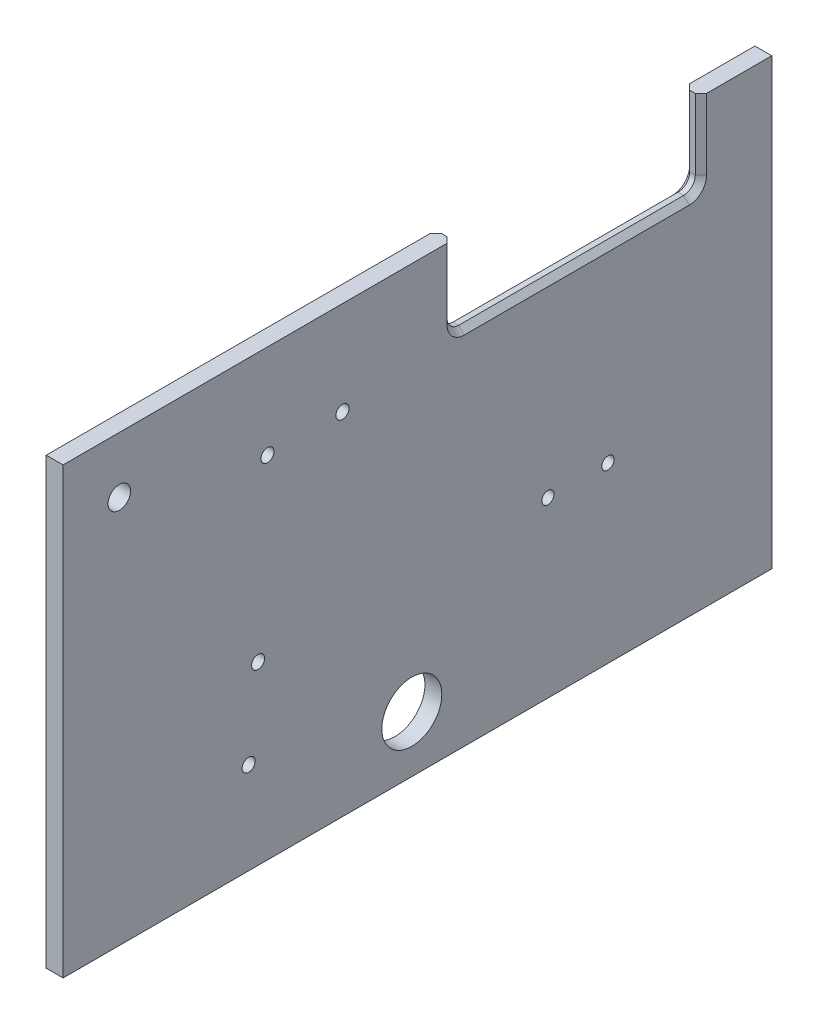
SolidWorks part; units mm, degrees
material "Q235-A"
ref_plane "Front Plane" through (0, 0, 0) normal (0, 0, 1) x (1, 0, 0)
ref_plane "Top Plane" through (0, 0, 0) normal (0, 1, 0) x (1, 0, 0)
ref_plane "Right Plane" through (0, 0, 0) normal (1, 0, 0) x (0, 0, -1)
sketch "Sketch1" plane through (0, 0, 0) normal (1, 0, 0) x (0, 0, -1)
  line L0 (0, -592.4523) -> (0, 592.4523) construction
  line L1 (0, 0) -> (520, 0)
  line L2 (520, 0) -> (520, 1185)
  line L3 (520, 1185) -> (331, 1185)
  line L4 (331, 1185) -> (331, 965)
  line L5 (331, 965) -> (-331, 965)
  line L6 (-331, 965) -> (-331, 1185)
  line L7 (-331, 1185) -> (-1370, 1185)
  line L8 (-1370, 1185) -> (-1370, 0)
  line L9 (-1370, 0) -> (0, 0)
  point P3 (0, 0)
  dimension "D1" = 1185
  dimension "D2" = 1890
  dimension "D3" = 520
  dimension "D4" = 662
  dimension "D5" = 220
extrude "Boss-Extrude1" add sketch "Sketch1" along normal mid plane 45
sketch "Sketch2" plane through (22.5, 0, 0) normal (1, 0, 0) x (0, 0, -1)
  line L0 (-331, 1185) -> (-1370, 1185) construction
  line L1 (-1370, 1185) -> (-1370, 0) construction
  line L2 (0, 0) -> (0, 260.9567) construction
  line L3 (-1370, 0) -> (520, 0) construction
  circle A0 centre (-1220, 1035) radius 30
  circle A1 centre (-825, 935) radius 17.5
  circle A2 centre (-625, 935) radius 17.5
  circle A3 centre (-850, 470) radius 17.5
  circle A4 centre (-875, 245) radius 17.5
  circle A5 centre (-440, 150) radius 80
  dimension "D1" = 150
  dimension "D2" = 150
  dimension "D3" = 60
  dimension "D4" = 495
  dimension "D5" = 25
  dimension "D6" = 25
  dimension "D7" = 200
  dimension "D8" = 35
  dimension "D9" = 250
  dimension "D10" = 465
  dimension "D11" = 225
  dimension "D12" = 440
  dimension "D13" = 150
  dimension "D14" = 160
extrude "Cut-Extrude1" cut sketch "Sketch2" against normal through all
fillet "Fillet1" radius 31 2 edges at (0, 965, -331) (0, 965, 331)
chamfer "Chamfer1" distance 15 angle 45 10 edges at (-22.5, 1090.5, 331) (-22.5, 974.0797, 321.9203) (-22.5, 965, 0) (-22.5, 974.0797, -321.9203) (-22.5, 1090.5, -331) (22.5, 1090.5, -331) (22.5, 974.0797, -321.9203) (22.5, 965, 0) (22.5, 974.0797, 321.9203) (22.5, 1090.5, 331)
sketch "Sketch3" plane through (22.5, 0, 0) normal (1, 0, 0) x (0, 0, -1)
  line L0 (0, 0) -> (0, 840.0935) construction
  line L1 (-77, 463) -> (83, 463) construction
  line L2 (-346, 1185) -> (-1370, 1185) construction
  circle A0 centre (-77, 463) radius 16.5
  circle A1 centre (83, 463) radius 16.5
  dimension "D1" = 160
  dimension "D2" = 33
  dimension "D3" = 77
  dimension "D4" = 722
extrude "Cut-Extrude2" cut sketch "Sketch3" against normal blind 159
